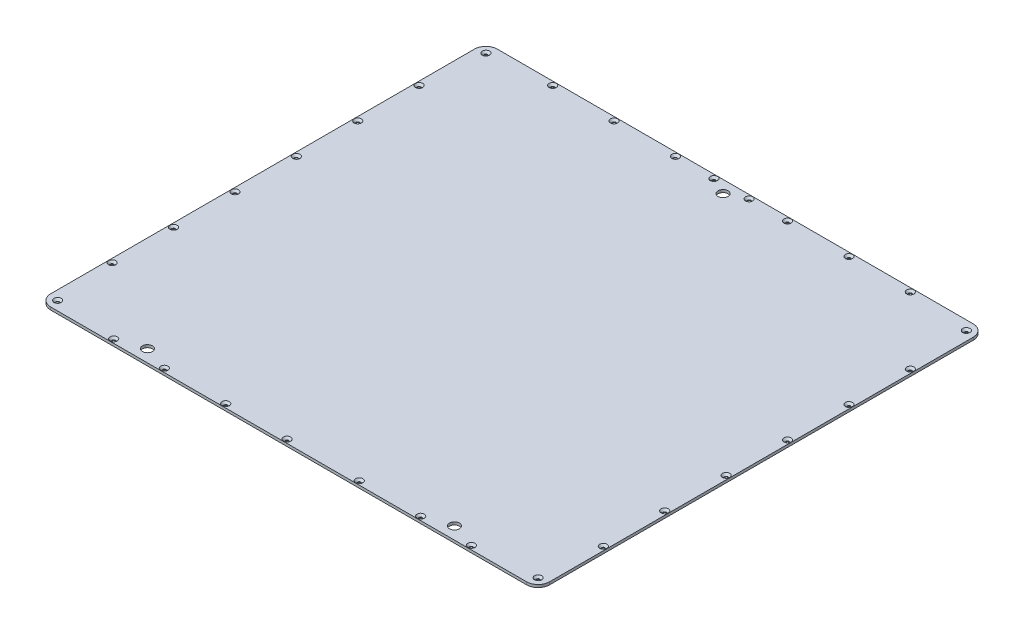
from build123d import *

# Parameters (mm, degrees)
BOSS_EXTRUDE1_DEPTH                             = 3.5
SKETCH2_R                                       = 6.5
CUT_EXTRUDE1_DEPTH                              = 437.254799401
CSK_FOR_M4_FLAT_HEAD_MACHINE_SCREW1_D           = 4.3
CSK_FOR_M4_FLAT_HEAD_MACHINE_SCREW1_DEPTH       = 7.5
CSK_FOR_M4_FLAT_HEAD_MACHINE_SCREW1_CSINK_D     = 9.4
CSK_FOR_M4_FLAT_HEAD_MACHINE_SCREW1_CSINK_ANGLE = 90
CSK_FOR_M4_FLAT_HEAD_MACHINE_SCREW1_TIP         = 1.291850331


with BuildPart() as part:
    # Sketch1 → Boss-Extrude1 (new body)
    with BuildSketch(Plane(origin=(0, 0, 0), x_dir=(1, 0, 0), z_dir=(0, 1, 0))):
        with BuildLine():
            Line((-310, -291), (310, -291))
            ThreePointArc((310, -291), (320.606601718, -286.606601718), (325, -276))
            Line((325, -276), (325, 276))
            ThreePointArc((325, 276), (320.606601718, 286.606601718), (310, 291))
            Line((310, 291), (-310, 291))
            ThreePointArc((-310, 291), (-320.606601718, 286.606601718), (-325, 276))
            Line((-325, 276), (-325, -276))
            ThreePointArc((-325, -276), (-320.606601718, -286.606601718), (-310, -291))
        make_face()
    extrude(amount=BOSS_EXTRUDE1_DEPTH)

    # Sketch2 → Cut-Extrude1 (cut, through all)
    with BuildSketch(Plane(origin=(0, 3.5, 0), x_dir=(1, 0, 0), z_dir=(0, 1, 0))):
        with Locations(Location((0, 275, 0), (0, 0, 270))):
            Circle(SKETCH2_R)
        with Locations(Location((200, -275, 0), (0, 0, 270))):
            Circle(SKETCH2_R)
        with Locations(Location((-200, -275, 0), (0, 0, 270))):
            Circle(SKETCH2_R)
    extrude(amount=-CUT_EXTRUDE1_DEPTH, mode=Mode.SUBTRACT)

    # CSK for M4 Flat Head Machine Screw1
    with Locations(Plane(origin=(0, 3.5, 0), x_dir=(1, 0, 0), z_dir=(0, 1, 0))):
        with Locations((-233, 286), (-313, 279), (-153, 286), (-73, 286), (-23, 286), (73, 286), (153, 286), (313, 279), (-320, 199), (-320, 119), (-320, 39), (-320, -41), (-320, -121), (-320, -201), (-313, -279), (-233, -286), (-167, -286), (-87, -286), (-7, -286), (87, -286), (167, -286), (313, -279), (320, -201), (320, -121), (320, -41), (320, 39), (320, 119), (320, 199), (233, 286), (23, 286), (233, -286)):
            CounterSinkHole(CSK_FOR_M4_FLAT_HEAD_MACHINE_SCREW1_D / 2, CSK_FOR_M4_FLAT_HEAD_MACHINE_SCREW1_CSINK_D / 2, depth=CSK_FOR_M4_FLAT_HEAD_MACHINE_SCREW1_DEPTH, counter_sink_angle=CSK_FOR_M4_FLAT_HEAD_MACHINE_SCREW1_CSINK_ANGLE)
            with Locations((0, 0, -(CSK_FOR_M4_FLAT_HEAD_MACHINE_SCREW1_DEPTH + CSK_FOR_M4_FLAT_HEAD_MACHINE_SCREW1_TIP / 2))):  # 118° drill point
                Cone(0, CSK_FOR_M4_FLAT_HEAD_MACHINE_SCREW1_D / 2, CSK_FOR_M4_FLAT_HEAD_MACHINE_SCREW1_TIP, mode=Mode.SUBTRACT)


solid = part.part
